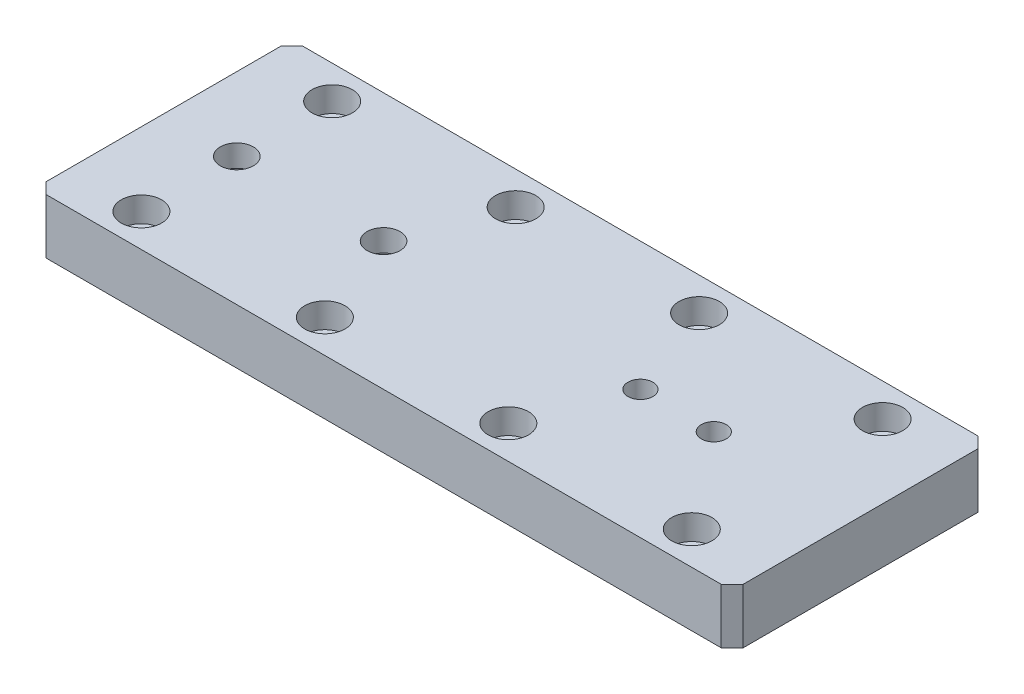
from build123d import *

# Parameters (mm, degrees)
SKETCH_1_W                = 190
SKETCH_1_H                = 70
EXTRUDE_1_DEPTH           = 15
CHAMFER_1_SIZE            = 3
HOLE_WIZARD_5_D           = 6.6
HOLE_WIZARD_5_CBORE_D     = 11
HOLE_WIZARD_5_CBORE_DEPTH = 6.8
HOLE_WIZARD_3_D           = 9
HOLE_WIZARD_3_CBORE_D     = 15
HOLE_WIZARD_3_CBORE_DEPTH = 9
HOLE_WIZARD_M8_1_D        = 6.8


with BuildPart() as part:
    # 草图1 → 凸台-拉伸1 (new body)
    with BuildSketch(Plane(origin=(0, 0, 0), x_dir=(1, 0, 0), z_dir=(0, 1, 0))):
        Rectangle(SKETCH_1_W, SKETCH_1_H)
    extrude(amount=EXTRUDE_1_DEPTH)

    # 倒角1
    chamfer_1_edges = [part.edges().sort_by_distance(p)[0] for p in [
        (95, 7.5, 35),
        (-95, 7.5, 35),
        (-95, 7.5, -35),
        (95, 7.5, -35),
    ]]
    chamfer(chamfer_1_edges, length=CHAMFER_1_SIZE)

    # 打孔尺寸(%根据)内六角圆柱头螺钉的类型5 (through all)
    with Locations(Plane(origin=(0, 15, 0), x_dir=(1, 0, 0), z_dir=(0, 1, 0))):
        with Locations((75, -26), (25, -26), (-25, -26), (-75, -26), (25, 26), (-25, 26), (-75, 26), (75, 26)):
            CounterBoreHole(HOLE_WIZARD_5_D / 2, HOLE_WIZARD_5_CBORE_D / 2, HOLE_WIZARD_5_CBORE_DEPTH)

    # 打孔尺寸(%根据)内六角圆柱头螺钉的类型3 (through all)
    with Locations(Plane(origin=(0, 0, 0), x_dir=(-1, 0, 0), z_dir=(0, -1, 0))):
        with Locations((35, 0), (75, 0)):
            CounterBoreHole(HOLE_WIZARD_3_D / 2, HOLE_WIZARD_3_CBORE_D / 2, HOLE_WIZARD_3_CBORE_DEPTH)

    # M8 螺纹孔1 (through all)
    with Locations(Plane(origin=(0, 15, 0), x_dir=(1, 0, 0), z_dir=(0, 1, 0))):
        with Locations((55, 0), (35, 0)):
            Hole(HOLE_WIZARD_M8_1_D / 2)


solid = part.part
